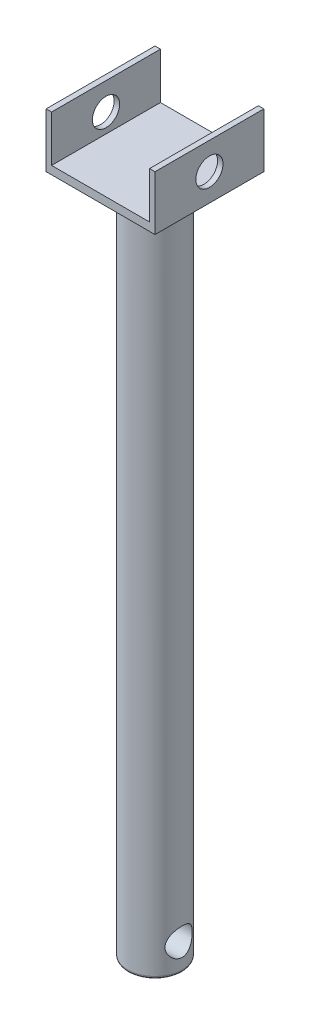
SolidWorks part; units mm, degrees
ref_plane "Front Plane" through (0, 0, 0) normal (0, 0, 1) x (1, 0, 0)
ref_plane "Top Plane" through (0, 0, 0) normal (0, 1, 0) x (1, 0, 0)
ref_plane "Right Plane" through (0, 0, 0) normal (1, 0, 0) x (0, 0, -1)
sketch "Sketch1" plane through (0, 0, 0) normal (0, 0, 1) x (1, 0, 0)
  line L0 (-180, 0) -> (180, 0)
  line L1 (180, 0) -> (180, 170)
  line L2 (180, 170) -> (200, 170)
  line L3 (200, 170) -> (200, -30)
  line L4 (200, -30) -> (-200, -30)
  line L5 (-200, -30) -> (-200, 170)
  line L6 (-200, 170) -> (-180, 170)
  line L7 (-180, 170) -> (-180, 0)
  dimension "D1" = 360
  dimension "D2" = 400
  dimension "D3" = 180
  dimension "D4" = 200
  dimension "D5" = 200
  dimension "D6" = 200
  dimension "D7" = 30
extrude "Boss-Extrude1" add sketch "Sketch1" along normal blind 400
sketch "Sketch2" plane through (200, 0, 0) normal (1, 0, 0) x (0, 0, -1)
  line L0 (0, -30) -> (0, 170) construction
  line L1 (-400, -30) -> (0, -30) construction
  circle A0 centre (-200, 70) radius 50
  dimension "D1" = 100
  dimension "D2" = 200
  dimension "D3" = 100
extrude "Cut-Extrude1" cut sketch "Sketch2" against normal blind 400
sketch "Sketch3" plane through (0, -30, 0) normal (0, -1, 0) x (1, 0, 0)
  line L0 (-200, 0) -> (200, 0) construction
  circle A0 centre (0, 200) radius 100
  dimension "D1" = 200
  dimension "D2" = 200
extrude "Boss-Extrude2" add sketch "Sketch3" along normal blind 2500
sketch "Sketch4" plane through (0, 0, 0) normal (1, 0, 0) x (0, 0, -1)
  line L0 (-300, -2530) -> (-100, -2530) construction
  line L1 (-100, -2530) -> (-100, -30) construction
  circle A0 centre (-200, -2430) radius 50
  dimension "D1" = 100
  dimension "D2" = 100
  dimension "D3" = 100
extrude "Cut-Extrude2" cut sketch "Sketch4" against normal blind 2500 and the other way blind 2500
fillet "Fillet1" radius 10 1 edges at (100, -2530, 200)
